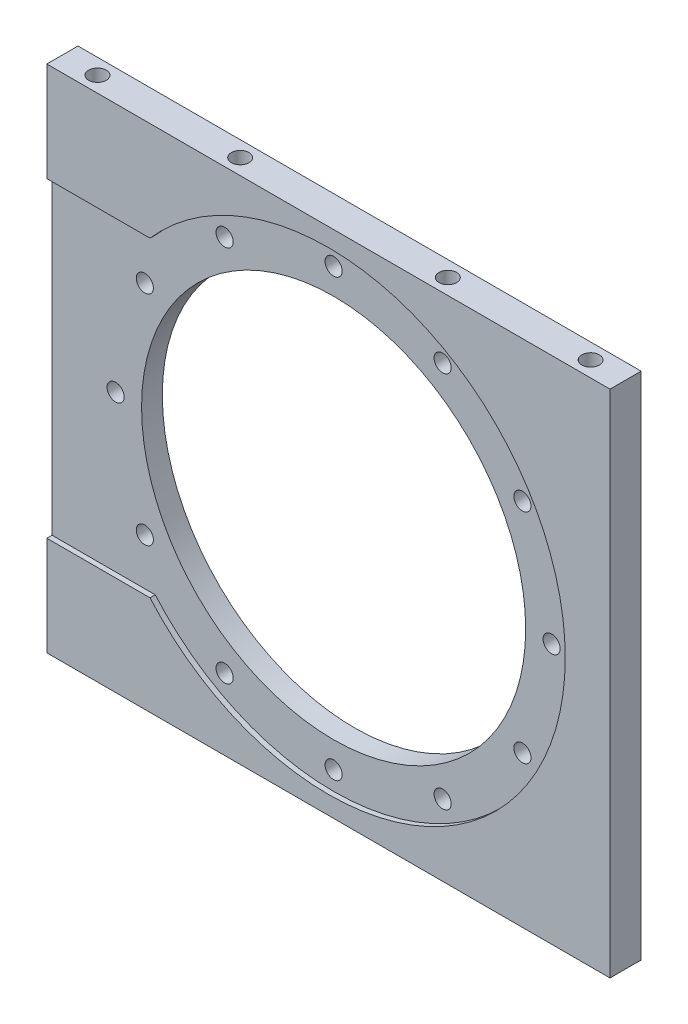
from build123d import *

# Parameters (mm, degrees)
SKETCH_1_W             = 217
SKETCH_1_H             = 196.5
SKETCH_1_R             = 74
EXTRUDE_1_DEPTH        = 12
SKETCH_2_R             = 91.25
CUT_EXTRUDE_1_DEPTH    = 2
CUT_EXTRUDE_START      = -2
SKETCH_3_R             = 91.25
CUT_EXTRUDE_2_DEPTH    = 2
SKETCH_4_W             = 39.75
SKETCH_4_H             = 120
CUT_EXTRUDE_3_DEPTH    = 2
HOLE_WIZARD_M6_1_D     = 6.6
HOLE_WIZARD_M8_1_D     = 6.8
HOLE_WIZARD_M8_1_DEPTH = 19.75
HOLE_WIZARD_M8_1_TIP   = 2.042926105
HOLE_WIZARD_M8_2_D     = 6.8
HOLE_WIZARD_M8_2_DEPTH = 19.75
HOLE_WIZARD_M8_2_TIP   = 2.042926105


with BuildPart() as part:
    # 草图1 → 凸台-拉伸1 (new body)
    with BuildSketch(Plane.XY):
        Rectangle(SKETCH_1_W, SKETCH_1_H)
        Circle(SKETCH_1_R, mode=Mode.SUBTRACT)
    extrude(amount=EXTRUDE_1_DEPTH)

    # 草图2 → 切除-拉伸1 (cut)
    with BuildSketch(Plane(origin=(0, 0, 0), x_dir=(-1, 0, 0), z_dir=(0, 0, -1))):
        Circle(SKETCH_2_R)
    extrude(amount=-CUT_EXTRUDE_1_DEPTH, mode=Mode.SUBTRACT)

    # 草图3 → 切除-拉伸2 (cut)
    with BuildSketch(Plane.XY.offset(12).offset(CUT_EXTRUDE_START)):
        with Locations(Location((0, 0, 0), (0, 0, 180))):
            Circle(SKETCH_3_R)
    extrude(amount=CUT_EXTRUDE_2_DEPTH, mode=Mode.SUBTRACT)

    # 草图4 → 切除-拉伸3 (cut)
    with BuildSketch(Plane.XY.offset(12)):
        with Locations((-88.625, 0)):
            Rectangle(SKETCH_4_W, SKETCH_4_H)
    extrude(amount=-CUT_EXTRUDE_3_DEPTH, mode=Mode.SUBTRACT)

    # M6 间隙孔1 (through all)
    with Locations(Plane(origin=(0, 0, 2), x_dir=(-1, 0, 0), z_dir=(0, 0, -1))):
        with Locations((0, 84), (42, 72.746133918), (72.746133918, 42), (84, 0), (72.746133918, -42), (42, -72.746133918), (0, -84), (-42, -72.746133918), (-72.746133918, -42), (-84, 0), (-72.746133918, 42), (-42, 72.746133918)):
            Hole(HOLE_WIZARD_M6_1_D / 2)

    # M8 螺纹孔1
    with Locations(Plane(origin=(0, -98.25, 0), x_dir=(-1, 0, 0), z_dir=(0, -1, 0))):
        with Locations((-95, -6), (-40, -6), (40, -6), (95, -6)):
            Hole(HOLE_WIZARD_M8_1_D / 2, depth=HOLE_WIZARD_M8_1_DEPTH)
            with Locations((0, 0, -(HOLE_WIZARD_M8_1_DEPTH + HOLE_WIZARD_M8_1_TIP / 2))):  # 118° drill point
                Cone(0, HOLE_WIZARD_M8_1_D / 2, HOLE_WIZARD_M8_1_TIP, mode=Mode.SUBTRACT)

    # M8 螺纹孔2
    with Locations(Plane(origin=(0, 98.25, 0), x_dir=(1, 0, 0), z_dir=(0, 1, 0))):
        with Locations((-95, -6), (-40, -6), (40, -6), (95, -6)):
            Hole(HOLE_WIZARD_M8_2_D / 2, depth=HOLE_WIZARD_M8_2_DEPTH)
            with Locations((0, 0, -(HOLE_WIZARD_M8_2_DEPTH + HOLE_WIZARD_M8_2_TIP / 2))):  # 118° drill point
                Cone(0, HOLE_WIZARD_M8_2_D / 2, HOLE_WIZARD_M8_2_TIP, mode=Mode.SUBTRACT)


solid = part.part
